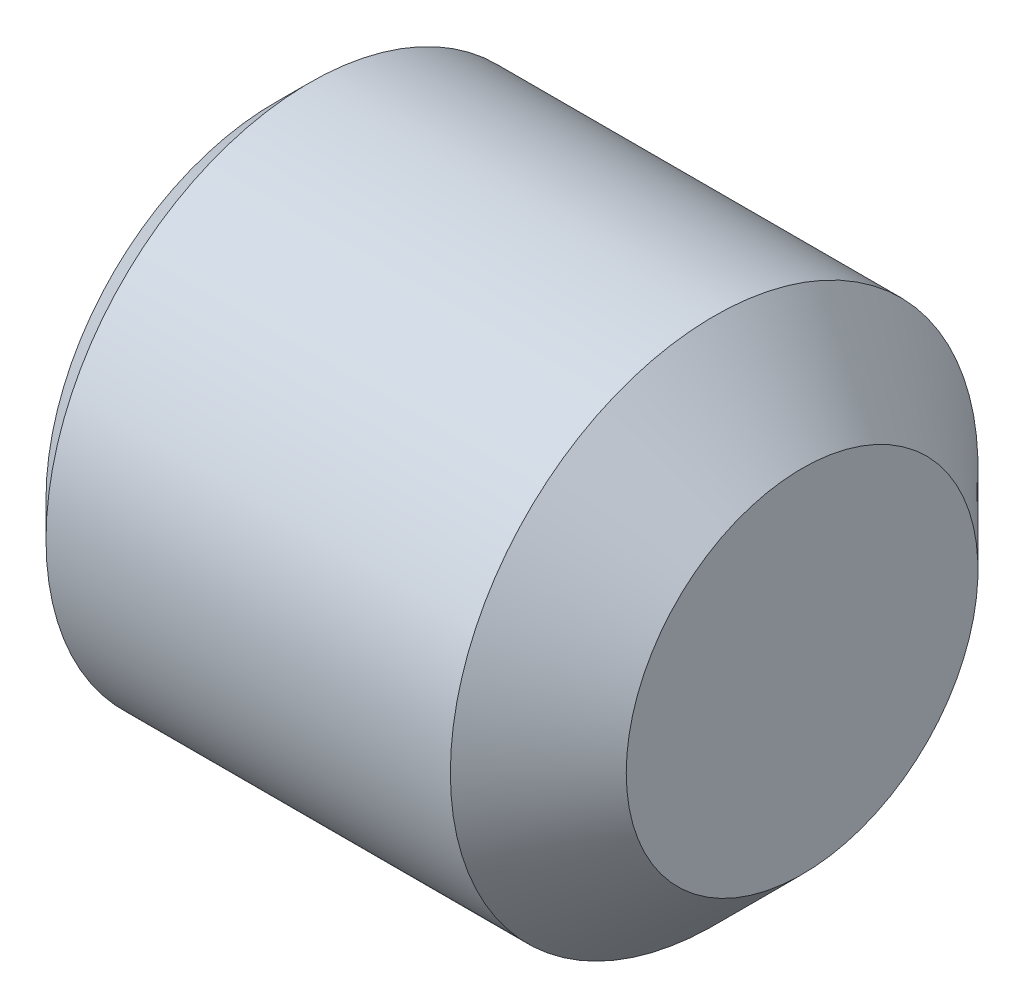
from build123d import *

# Parameters (mm, degrees)
CUT_EXTRUDE1_DEPTH = 1.2


with BuildPart() as part:
    # Sketch1 → Base-Revolve (revolve)
    with BuildSketch(Plane.XY, mode=Mode.PRIVATE) as base_revolve_sk:
        Polygon((0, 0), (3, 0), (3, 1), (2.5, 1.5), (0.201, 1.5), (0, 1.299), align=None)
    revolve(base_revolve_sk.sketch.rotate(Axis((-0.277777778, 0, 0), (1, 0, 0)), 90), axis=Axis((-0.277777778, 0, 0), (1, 0, 0)))

    # Sketch2 → Cut-Extrude1 (cut)
    with BuildSketch(Plane.ZY):
        Polygon((-0.4325, -0.749111974), (0.4325, -0.749111974), (0.865, 0), (0.4325, 0.749111974), (-0.4325, 0.749111974), (-0.865, 0), align=None)
    extrude(amount=-CUT_EXTRUDE1_DEPTH, mode=Mode.SUBTRACT)

    # Sketch4 → Cut-Revolve2 (revolve, cut)
    with BuildSketch(Plane.XY, mode=Mode.PRIVATE) as cut_revolve2_sk:
        Polygon((1.2, 0.749111974), (1.6325, 0), (1.2, 0), align=None)
    revolve(cut_revolve2_sk.sketch.rotate(Axis((-0.277777778, 0, 0), (1, 0, 0)), 90), axis=Axis((-0.277777778, 0, 0), (1, 0, 0)), mode=Mode.SUBTRACT)


solid = part.part
